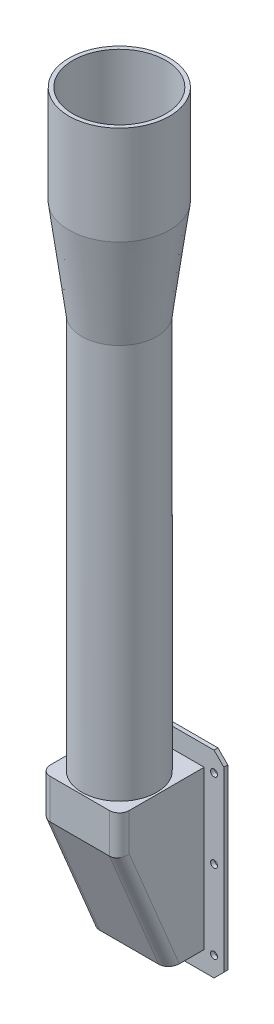
SolidWorks part; units mm, degrees
ref_plane "Front Plane" through (0, 0, 0) normal (0, 0, 1) x (1, 0, 0)
ref_plane "Top Plane" through (0, 0, 0) normal (0, 1, 0) x (1, 0, 0)
ref_plane "Right Plane" through (0, 0, 0) normal (1, 0, 0) x (0, 0, -1)
sketch "Sketch1" plane through (0, 0, 0) normal (0, 0, 1) x (1, 0, 0)
  line L1 (-20, 40) -> (20, 40)
  line L2 (-20, 40) -> (-20, -40)
  line L3 (-20, -40) -> (20, -40)
  line L4 (20, 40) -> (20, -40)
  line L5 (-20, 40) -> (20, -40) construction
  line L6 (-20, -40) -> (20, 40) construction
  point P0 (0, 0)
  dimension "D1" = 80
  dimension "D2" = 40
extrude "Boss-Extrude1" add sketch "Sketch1" along normal blind 45
sketch "Sketch2" plane through (0, 40, 0) normal (0, 1, 0) x (1, 0, 0)
  line L1 (20, -45) -> (-20, -45) construction
  circle A0 centre (0, -25) radius 19
  dimension "D1" = 38
  dimension "D2" = 20
extrude "Boss-Extrude2" add sketch "Sketch2" along normal blind 200
sketch "Sketch3" plane through (20, 0, 0) normal (1, 0, 0) x (0, 0, -1)
  line L0 (-20, -40) -> (-45, 20)
  line L1 (-45, -40) -> (0, -40) construction
  line L2 (-45, -40) -> (-45, 40) construction
  line L3 (0, -40) -> (0, 40) construction
  line L4 (-45, 40) -> (0, 40) construction
  dimension "D1" = 20
  dimension "D2" = 20
extrude "Cut-Extrude1" cut sketch "Sketch3" against normal through all and the other way through all
shell "Shell1" thickness 2
sketch "Sketch4" plane through (0, 0, 0) normal (0, 0, -1) x (-1, 0, 0)
  line L0 (-20, -40) -> (-20, 40) construction
  line L1 (-30, -50) -> (30, -50)
  line L2 (-30, -50) -> (-30, 50)
  line L3 (-30, 50) -> (30, 50)
  line L4 (30, -50) -> (30, 50)
  line L5 (-30, -50) -> (30, 50) construction
  line L6 (-30, 50) -> (30, -50) construction
  line L8 (20, 40) -> (20, -40) construction
  line L9 (-20, -40) -> (-20, 40)
  line L10 (20, 40) -> (20, -40)
  line L11 (-20, 40) -> (20, 40) construction
  point P0 (0, 0)
  line M5 (-20, 40) -> (-20, -40)
  line M7 (20, -40) -> (20, 40)
  dimension "D1" = 10
  dimension "D2" = 10
extrude "Boss-Extrude3" add sketch "Sketch4" against normal blind 2 contours L3 L2 L1 M5 | L1 L4 L3 M7
chamfer "Chamfer1" distance 5 angle 45 4 edges at (-30, 50, 1) (30, 50, 1) (30, -50, 1) (-30, -50, 1)
sketch "Sketch5" plane through (0, 0, 2) normal (0, 0, 1) x (1, 0, 0)
  line L1 (-30, -45) -> (-30, 45) construction
  circle A0 centre (-25, 0) radius 1.75
  circle A3 centre (-25, 40) radius 1.75
  circle A4 centre (-25, -40) radius 1.75
  dimension "D1" = 5
  dimension "D2" = 3.5
  dimension "D3" = 40
  dimension "D4" = 80
extrude "Cut-Extrude2" cut sketch "Sketch5" against normal blind 10
mirror "Mirror1" about plane through (0, 0, 0) normal (1, 0, 0) of "Cut-Extrude2"
sketch "Sketch6" plane through (0, 0, 2) normal (0, 0, 1) x (1, 0, 0)
  line L0 (25, -50) -> (-25, -50) construction
  circle A0 centre (0, -45) radius 1.75
  dimension "D1" = 3.5
  dimension "D2" = 5
extrude "Cut-Extrude3" cut sketch "Sketch6" against normal blind 10
sketch "Sketch7" plane through (0, 0, 0) normal (1, 0, 0) x (0, 0, -1)
  line L0 (-44, 240) -> (-50.5, 290)
  line L1 (-50.5, 290) -> (-50.5, 340)
  line L2 (-50.5, 340) -> (-48.5, 340)
  line L3 (-25, 340) -> (-25, 240)
  line L4 (-6, 240) -> (-44, 240) construction
  line L5 (-41.9832, 240) -> (-44, 240)
  line L6 (-48.5, 290.1295) -> (-48.5, 340)
  line L7 (-48.5, 290.1295) -> (-48.5, 338) construction
  line L9 (-42.2432, 242) -> (-48.5, 290.1295) construction
  line L10 (-41.9832, 240) -> (-48.5, 290.1295)
  line L11 (-48.5, 338) -> (-27, 338) construction
  line L12 (-27, 242) -> (-42.2432, 242) construction
  line L13 (-27, 338) -> (-27, 242) construction
  line L14 (-25, 240) -> (-44, 240) construction
  line L15 (-50.5, 340) -> (-25, 340) construction
  dimension "D1" = 50
  dimension "D2" = 50
  dimension "D3" = 25.5
  dimension "D4" = 2
revolve "Revolve1" add sketch "Sketch7" angle 360 about L3
fillet "Fillet1" radius 5 4 edges at (-20, -10, 32.5) (-20, 30, 45) (20, -10, 32.5) (20, 30, 45)
